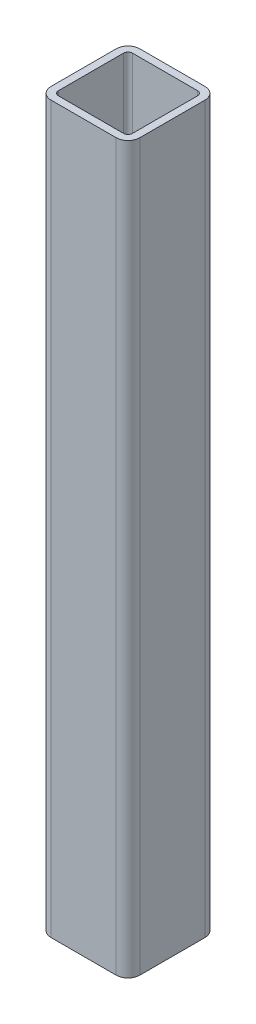
SolidWorks part; units mm, degrees
material "XRAAT"
ref_plane "前视基准面" through (0, 0, 0) normal (0, 0, 1) x (1, 0, 0)
ref_plane "上视基准面" through (0, 0, 0) normal (0, 1, 0) x (1, 0, 0)
ref_plane "右视基准面" through (0, 0, 0) normal (1, 0, 0) x (0, 0, -1)
sketch "草图1" plane through (0, 0, 0) normal (0, 0, 1) x (1, 0, 0)
  line L0 (0, 0) -> (0, 980)
  dimension "D1" = 980
other "结构用冷弯空心方钢(gb t6728-2002) 120×120×10(1)"
ref_plane "基准面1" through (0, 0, 0) normal (0, 1, 0) x (-1, 0, 0)
sketch "Sketch12" plane through (0, 0, 0) normal (0, 1, 0) x (-1, 0, 0)
  line L0 (-44, -50) -> (44, -50)
  line L1 (-50, -44) -> (-50, 44)
  line L2 (44, 50) -> (-44, 50)
  line L3 (50, 44) -> (50, -44)
  line L4 (-44, -60) -> (44, -60)
  line L5 (-60, -44) -> (-60, 44)
  line L6 (44, 60) -> (-44, 60)
  line L7 (60, 44) -> (60, -44)
  arc A0 (60, 44) -> (44, 60) centre (44, 44) ccw
  arc A1 (44, -60) -> (60, -44) centre (44, -44) ccw
  arc A2 (-60, -44) -> (-44, -60) centre (-44, -44) ccw
  arc A3 (-44, 60) -> (-60, 44) centre (-44, 44) ccw
  arc A4 (-44, 50) -> (-50, 44) centre (-44, 44) ccw
  arc A5 (50, 44) -> (44, 50) centre (44, 44) ccw
  arc A6 (44, -50) -> (50, -44) centre (44, -44) ccw
  arc A7 (-50, -44) -> (-44, -50) centre (-44, -44) ccw
  point P0 (-60, 0)
  point P1 (60, 0)
  point P2 (0, 60)
  point P3 (0, -60)
  point P4 (0, 0)
  point P5 (-60, -60)
  point P6 (60, -60)
  point P7 (60, 60)
  point P8 (-60, 60)
  point P33 (0, 0)
  dimension "D1" = 16
  dimension "D2" = 120
  dimension "D3" = 10
